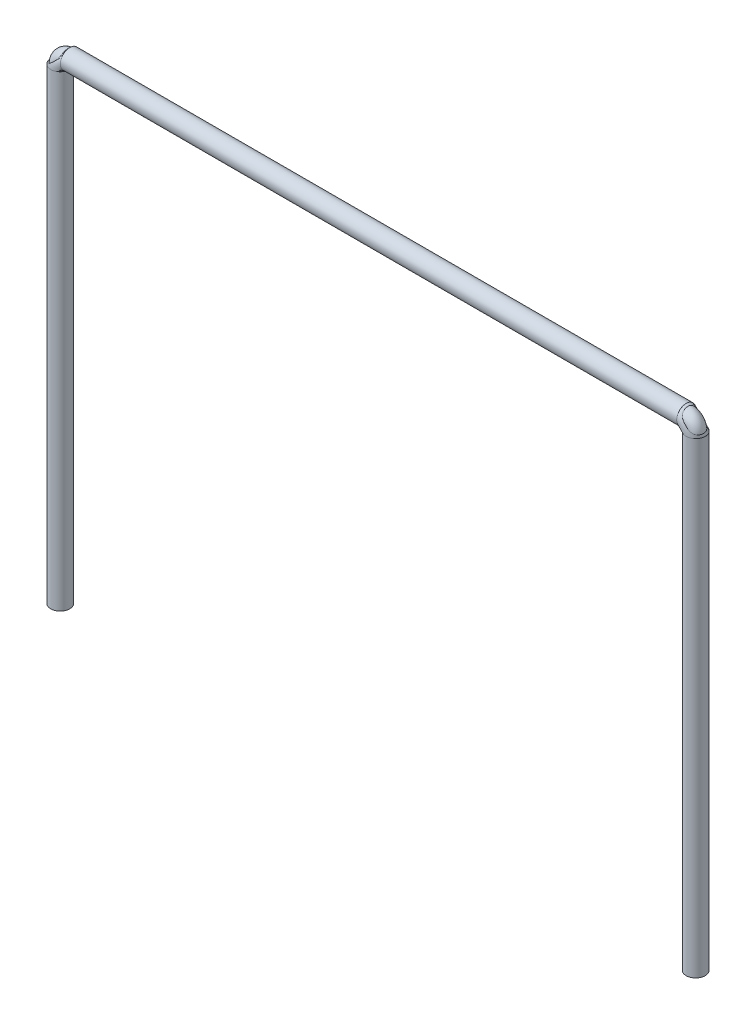
from build123d import *

# Parameters (mm, degrees)
SKETCH1_R                                  = 30
SKETCH1_R_2                                = 25
GB_T6728_2002_ROUND_TUBE_060_X_5_1_DEPTH   = 1470
SKETCH1_ON_SEGMENT_2_R                     = 30
SKETCH1_ON_SEGMENT_2_R_2                   = 25
GB_T6728_2002_ROUND_TUBE_060_X_5_1_2_ANGLE = 90
SKETCH1_ON_SEGMENT_3_R                     = 30
SKETCH1_ON_SEGMENT_3_R_2                   = 25
GB_T6728_2002_ROUND_TUBE_060_X_5_1_3_DEPTH = 1940
SKETCH1_ON_SEGMENT_4_R                     = 30
SKETCH1_ON_SEGMENT_4_R_2                   = 25
GB_T6728_2002_ROUND_TUBE_060_X_5_1_4_ANGLE = 90
SKETCH1_ON_SEGMENT_5_R                     = 30
SKETCH1_ON_SEGMENT_5_R_2                   = 25
GB_T6728_2002_ROUND_TUBE_060_X_5_1_5_DEPTH = 1470


with BuildPart() as part:
    # Sketch1 → Gb／t6728-2002 round tube 060 X 5 (1) (new body)
    with BuildSketch(Plane(origin=(0, 0, 0), x_dir=(1, 0, 0), z_dir=(0, 1, 0))):
        Circle(SKETCH1_R)
        Circle(SKETCH1_R_2, mode=Mode.SUBTRACT)
    extrude(amount=GB_T6728_2002_ROUND_TUBE_060_X_5_1_DEPTH)


with BuildPart() as body_2:
    # Sketch1 on segment 2 (carried to the start of arc 2) → Gb_t6728-2002 round tube 060 X 5 _1 2 (revolve)
    with BuildSketch(Plane(origin=(0, 1470, 0), x_dir=(1, 0, 0), z_dir=(0, 1, 0))):
        Circle(SKETCH1_ON_SEGMENT_2_R)
        Circle(SKETCH1_ON_SEGMENT_2_R_2, mode=Mode.SUBTRACT)
    revolve(axis=Axis((30, 1470, 0), (0, 0, -1)), revolution_arc=GB_T6728_2002_ROUND_TUBE_060_X_5_1_2_ANGLE)


with BuildPart() as body_3:
    # Sketch1 on segment 3 (carried to segment 3) → Gb_t6728-2002 round tube 060 X 5 _1 3 (new body)
    with BuildSketch(Plane(origin=(30, 1500, 0), x_dir=(0, -1, 0), z_dir=(1, 0, 0))):
        Circle(SKETCH1_ON_SEGMENT_3_R)
        Circle(SKETCH1_ON_SEGMENT_3_R_2, mode=Mode.SUBTRACT)
    extrude(amount=GB_T6728_2002_ROUND_TUBE_060_X_5_1_3_DEPTH)


with BuildPart() as body_4:
    # Sketch1 on segment 4 (carried to the start of arc 4) → Gb_t6728-2002 round tube 060 X 5 _1 4 (revolve)
    with BuildSketch(Plane(origin=(2000, 1470, 0), x_dir=(1, 0, 0), z_dir=(0, 1, 0))):
        Circle(SKETCH1_ON_SEGMENT_4_R)
        Circle(SKETCH1_ON_SEGMENT_4_R_2, mode=Mode.SUBTRACT)
    revolve(axis=Axis((1970, 1470, 0), (0, 0, 1)), revolution_arc=GB_T6728_2002_ROUND_TUBE_060_X_5_1_4_ANGLE)


with BuildPart() as body_5:
    # Sketch1 on segment 5 (carried to segment 5) → Gb_t6728-2002 round tube 060 X 5 _1 5 (new body)
    with BuildSketch(Plane(origin=(2000, 0, 0), x_dir=(1, 0, 0), z_dir=(0, 1, 0))):
        Circle(SKETCH1_ON_SEGMENT_5_R)
        Circle(SKETCH1_ON_SEGMENT_5_R_2, mode=Mode.SUBTRACT)
    extrude(amount=GB_T6728_2002_ROUND_TUBE_060_X_5_1_5_DEPTH)


solid = Compound([part.part, body_2.part, body_3.part, body_4.part, body_5.part])
